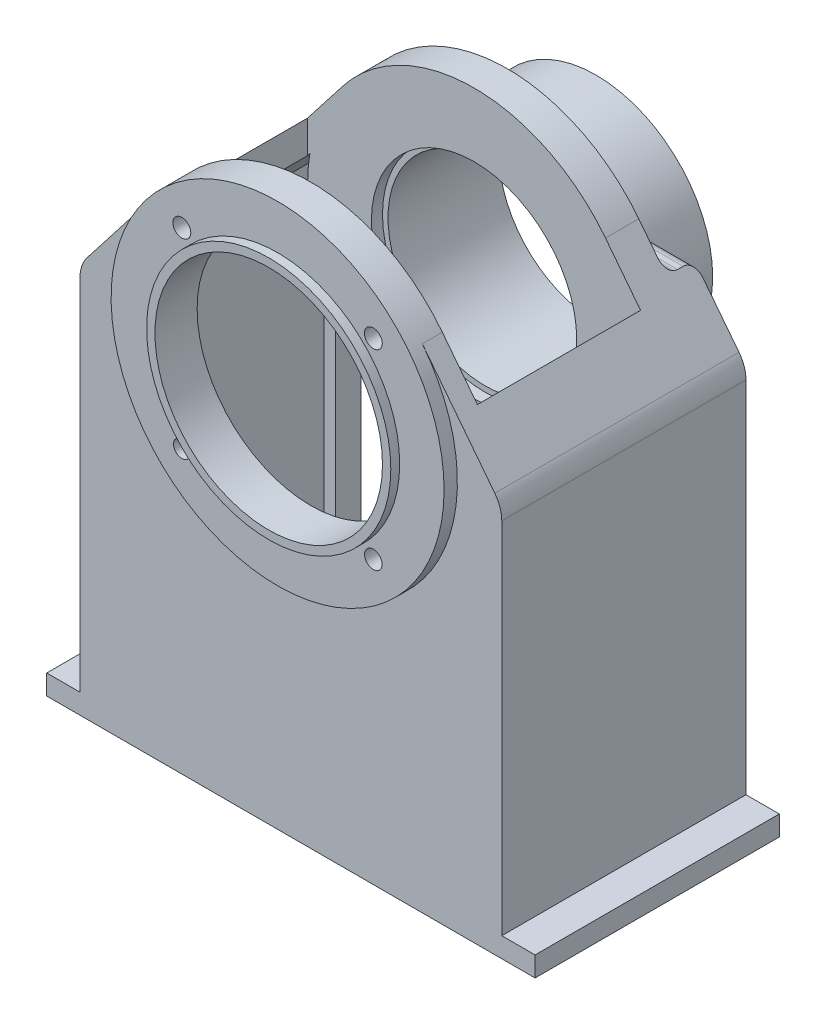
from build123d import *

# Parameters (mm, degrees)
BOSS_EXTRUDE1_DEPTH               = 7
SKETCH2_W                         = 48
SKETCH2_H                         = 7
BOSS_EXTRUDE2_DEPTH               = 352
SKETCH3_W                         = 18
SKETCH3_H                         = 7
BOSS_EXTRUDE3_DEPTH               = 352
BOSS_EXTRUDE4_DEPTH               = 18
BOSS_EXTRUDE5_START               = 30
BOSS_EXTRUDE5_DEPTH               = 30
BOSS_EXTRUDE6_DEPTH               = 147
BOSS_EXTRUDE7_DEPTH               = 147
BOSS_EXTRUDE8_START               = 18
BOSS_EXTRUDE8_DEPTH               = 18
SKETCH9_W                         = 30
SKETCH9_H                         = 220
CUT_EXTRUDE1_DEPTH                = 334
CUT_EXTRUDE2_DEPTH                = 30
CUT_EXTRUDE3_DEPTH                = 30
SKETCH12_W                        = 220
SKETCH12_H                        = 18
BOSS_EXTRUDE9_DEPTH               = 30
BOSS_EXTRUDE10_START              = 12
SKETCH13_R                        = 150
BOSS_EXTRUDE10_DEPTH              = 12
CUT_EXTRUDE4_DEPTH                = 37
SKETCH15_W                        = 340
SKETCH15_H                        = 240.614252285
BOSS_EXTRUDE11_DEPTH              = 5
CUT_EXTRUDE5_REACH                = 915.869
SKETCH16_W                        = 324
SKETCH16_H                        = 232.614252285
CUT_EXTRUDE6_DEPTH                = 25
SKETCH18_R                        = 110
BOSS_EXTRUDE12_DEPTH              = 8
SKETCH19_W                        = 105
SKETCH19_H                        = 80
HOLE1_D                           = 205
HOLE1_DEPTH                       = 38
M10_COUNTERBORE_HOLE1_D           = 12
M10_COUNTERBORE_HOLE1_DEPTH       = 45
M10_COUNTERBORE_HOLE1_CBORE_D     = 18
M10_COUNTERBORE_HOLE1_CBORE_DEPTH = 12
HOLE2_D                           = 175
HOLE2_CBORE_D                     = 185
HOLE2_CBORE_DEPTH                 = 10
FILLET1_R                         = 10
FILLET2_R                         = 18
FILLET3_R                         = 30
FILLET4_R                         = 150
SKETCH26_R                        = 8.054998693
SKETCH26_R_2                      = 7.927703382
SKETCH26_R_3                      = 7.509574851
CUT_EXTRUDE8_DEPTH                = 41


with BuildPart() as part:
    # Sketch1 → Boss-Extrude1 (new body)
    with BuildSketch(Plane.XY.offset(-1277.692981355)):
        with BuildLine():
            Line((671.230642584, 234.743963655), (711.230642584, 234.743963655))
            Line((711.230642584, 234.743963655), (521.230642584, 479.129447483))
            Line((521.230642584, 479.129447483), (331.230642584, 234.743963655))
            Line((331.230642584, 234.743963655), (371.230642584, 234.743963655))
            ThreePointArc((371.230642584, 234.743963655), (521.230642584, 84.743963655), (671.230642584, 234.743963655))
        make_face()
    extrude(amount=-BOSS_EXTRUDE1_DEPTH)

    # Sketch2 → Boss-Extrude2 (add)
    with BuildSketch(Plane.XZ.offset(-234.743963655)):
        with Locations((717.230642584, -1281.192981355)):
            Rectangle(SKETCH2_W, SKETCH2_H)
    extrude(amount=BOSS_EXTRUDE2_DEPTH)

    # Sketch3 → Boss-Extrude3 (add)
    with BuildSketch(Plane.XZ.offset(-234.743963654)):
        with Locations((340.230642584, -1281.192981355)):
            Rectangle(SKETCH3_W, SKETCH3_H)
    extrude(amount=BOSS_EXTRUDE3_DEPTH)

    # Sketch4 → Boss-Extrude4 (add)
    with BuildSketch(Plane(origin=(0, 0, -1284.692981355), x_dir=(-1, 0, 0), z_dir=(0, 0, -1))):
        Polygon((-331.230642584, -117.256036345), (-741.230642584, -117.256036345), (-741.230642584, 234.743963655), (-711.230642584, 234.743963655), (-521.230642584, 479.129447483), (-331.230642584, 234.743963655), align=None)
    extrude(amount=BOSS_EXTRUDE4_DEPTH)

    # Sketch5 → Boss-Extrude5 (add)
    with BuildSketch(Plane.XY.offset(-1277.692981355).offset(BOSS_EXTRUDE5_START)):
        with BuildLine():
            Line((371.230642584, 234.743963655), (354.030642584, 234.743963655))
            Line((354.030642584, 234.743963655), (349.230642584, 228.570014589))
            Line((349.230642584, 228.570014589), (349.230642584, -117.256036345))
            Line((349.230642584, -117.256036345), (331.230642584, -117.256036345))
            Line((331.230642584, -117.256036345), (331.230642584, 234.743963655))
            Line((331.230642584, 234.743963655), (521.230642584, 479.129447483))
            Line((521.230642584, 479.129447483), (711.230642584, 234.743963655))
            Line((711.230642584, 234.743963655), (741.230642584, 234.743963655))
            Line((741.230642584, 234.743963655), (741.230642584, -117.256036345))
            Line((741.230642584, -117.256036345), (693.230642584, -117.256036345))
            Line((693.230642584, -117.256036345), (693.230642584, 228.570014589))
            Line((693.230642584, 228.570014589), (688.430642584, 234.743963655))
            Line((688.430642584, 234.743963655), (671.230642584, 234.743963655))
            ThreePointArc((671.230642584, 234.743963655), (521.230642584, 84.743963655), (371.230642584, 234.743963655))
        make_face()
    extrude(amount=-BOSS_EXTRUDE5_DEPTH)

    # Sketch6 → Boss-Extrude6 (add)
    with BuildSketch(Plane.XY.offset(-1247.692981355)):
        Polygon((371.230642584, 256.867281138), (349.230642584, 228.570014589), (349.230642584, -117.256036345), (331.230642584, -117.256036345), (331.230642584, 234.743963655), (371.230642584, 286.193539197), align=None)
    extrude(amount=BOSS_EXTRUDE6_DEPTH)

    # Sketch7 → Boss-Extrude7 (add)
    with BuildSketch(Plane.XY.offset(-1247.692981355)):
        Polygon((741.230642584, -117.256036345), (693.230642584, -117.256036345), (693.230642584, 228.570014589), (671.230642584, 256.867281138), (671.230642584, 286.193539197), (711.230642584, 234.743963655), (741.230642584, 234.743963655), align=None)
    extrude(amount=BOSS_EXTRUDE7_DEPTH)

    # Sketch8 → Boss-Extrude8 (add)
    with BuildSketch(Plane.XY.offset(-1100.692981355).offset(BOSS_EXTRUDE8_START)):
        with BuildLine():
            Line((331.230642584, -117.256036345), (331.230642584, 234.743963654))
            Line((331.230642584, 234.743963654), (402.809589953, 326.811625152))
            ThreePointArc((402.809589953, 326.811625152), (521.230642584, 384.743963654), (639.651695216, 326.811625152))
            Line((639.651695216, 326.811625152), (711.230642584, 234.743963654))
            Line((711.230642584, 234.743963654), (741.230642584, 234.743963654))
            Line((741.230642584, 234.743963654), (741.230642584, -117.256036345))
            Line((741.230642584, -117.256036345), (331.230642584, -117.256036345))
        make_face()
    extrude(amount=-BOSS_EXTRUDE8_DEPTH)

    # Sketch9 → Cut-Extrude1 (cut)
    with BuildSketch(Plane(origin=(0, 234.743963655, 0), x_dir=(-1, 0, 0), z_dir=(0, 1, 0))):
        with Locations((-726.230642584, -1192.692981355)):
            Rectangle(SKETCH9_W, SKETCH9_H)
    extrude(amount=-CUT_EXTRUDE1_DEPTH, mode=Mode.SUBTRACT)

    # Sketch10 → Cut-Extrude2 (cut)
    with BuildSketch(Plane.XY.offset(-1247.692981355)):
        with BuildLine():
            Line((671.230642584, 234.743963655), (688.430642584, 234.743963655))
            Line((688.430642584, 234.743963655), (669.170885211, 259.516622202))
            ThreePointArc((669.170885211, 259.516622202), (670.714816319, 247.173034536), (671.230642584, 234.743963655))
        make_face()
    extrude(amount=-CUT_EXTRUDE2_DEPTH, mode=Mode.SUBTRACT)

    # Sketch11 → Cut-Extrude3 (cut)
    with BuildSketch(Plane.XY.offset(-1247.692981355)):
        with BuildLine():
            Line((373.290399958, 259.516622202), (354.030642584, 234.743963655))
            Line((354.030642584, 234.743963655), (371.230642584, 234.743963655))
            ThreePointArc((371.230642584, 234.743963655), (371.74646885, 247.173034536), (373.290399958, 259.516622202))
        make_face()
    extrude(amount=-CUT_EXTRUDE3_DEPTH, mode=Mode.SUBTRACT)

    # Sketch12 → Boss-Extrude9 (add)
    with BuildSketch(Plane.ZY.offset(-331.230642584)):
        with Locations((-1192.692981355, -108.256036346)):
            Rectangle(SKETCH12_W, SKETCH12_H)
    extrude(amount=BOSS_EXTRUDE9_DEPTH)

    # Sketch13 → Boss-Extrude10 (add)
    with BuildSketch(Plane.XY.offset(-1082.692981355).offset(BOSS_EXTRUDE10_START)):
        with Locations(Location((521.230642584, 234.743963655, 0), (0, 0, 142.136353638))):
            Circle(SKETCH13_R)
    extrude(amount=-BOSS_EXTRUDE10_DEPTH)

    # Sketch14 → Cut-Extrude4 (cut)
    with BuildSketch(Plane.XY.offset(-1247.692981355)):
        with BuildLine():
            Line((412.819587994, 184.743963655), (379.809286347, 184.743963655))
            ThreePointArc((379.809286347, 184.743963655), (521.230642584, 84.743963655), (662.651998822, 184.743963655))
            Line((662.651998822, 184.743963655), (629.641697174, 184.743963655))
            ThreePointArc((629.641697174, 184.743963655), (521.230642584, 115.35821594), (412.819587994, 184.743963655))
        make_face()
    extrude(amount=-CUT_EXTRUDE4_DEPTH, mode=Mode.SUBTRACT)

    # Sketch15 → Boss-Extrude11 (add)
    with BuildSketch(Plane(origin=(0, 0, -1302.692981355), x_dir=(-1, 0, 0), z_dir=(0, 0, -1))):
        with Locations((-521.230642584, 3.051089797)):
            Rectangle(SKETCH15_W, SKETCH15_H)
    extrude(amount=BOSS_EXTRUDE11_DEPTH)

    # Sketch16 → Cut-Extrude5 (cut, up to next)
    with BuildSketch(Plane(origin=(0, 0, -1307.692981355), x_dir=(-1, 0, 0), z_dir=(0, 0, -1)), mode=Mode.PRIVATE) as cut_extrude5_sk1:
        with Locations((-521.230642584, -0.948910203)):
            Rectangle(SKETCH16_W, SKETCH16_H)
    cut_extrude5_tool1 = extrude(cut_extrude5_sk1.sketch, amount=-CUT_EXTRUDE5_REACH, mode=Mode.PRIVATE) & part.part
    add(cut_extrude5_tool1.solids().sort_by_distance((521.230643, -0.94891, -1307.692981))[0], mode=Mode.SUBTRACT)

    # Sketch17 → Cut-Extrude6 (cut)
    with BuildSketch(Plane(origin=(0, 0, -1302.692981355), x_dir=(-1, 0, 0), z_dir=(0, 0, -1))):
        Polygon((-521.230642584, 479.129447483), (-664.583027426, 294.743963655), (-377.878257743, 294.743963655), align=None)
    extrude(amount=-CUT_EXTRUDE6_DEPTH, mode=Mode.SUBTRACT)

    # Sketch18 → Boss-Extrude12 (add)
    with BuildSketch(Plane.XY.offset(-1070.692981355)):
        with Locations((521.230642584, 234.743963655)):
            Circle(SKETCH18_R)
    extrude(amount=BOSS_EXTRUDE12_DEPTH)

    # Sketch19 → Revolve1 (revolve)
    with BuildSketch(Plane(origin=(280.2795082, 402.520798349, 0), x_dir=(-0.8206518066482866, 0.5714285714285761, 0), z_dir=(0.5714285714285761, 0.8206518066482866, 0)), mode=Mode.PRIVATE) as revolve1_sk:
        with Locations((-241.109460715, -1317.692981355)):
            Rectangle(SKETCH19_W, SKETCH19_H)
    revolve(revolve1_sk.sketch.rotate(Axis((521.230642584, 234.743963655, -1277.692981355), (0, 0, -1)), 325.150095421), axis=Axis((521.230642584, 234.743963655, -1277.692981355), (0, 0, -1)))

    # Hole1
    with Locations(Plane.XY.offset(-1062.692981355)):
        with Locations((521.230642584, 234.743963655)):
            Hole(HOLE1_D / 2, depth=HOLE1_DEPTH)

    # M10 counterbore hole1
    with Locations(Plane(origin=(0, 0, -1357.692981355), x_dir=(-1, 0, 0), z_dir=(0, 0, -1))):
        with Locations((-614.830642584, 234.743963655), (-521.230642584, 141.143963655), (-427.630642584, 234.743963655), (-521.230642584, 328.343963655)):
            CounterBoreHole(M10_COUNTERBORE_HOLE1_D / 2, M10_COUNTERBORE_HOLE1_CBORE_D / 2, M10_COUNTERBORE_HOLE1_CBORE_DEPTH, depth=M10_COUNTERBORE_HOLE1_DEPTH)

    # Hole2 (through all)
    with Locations(Plane.XY.offset(-1247.692981355)):
        with Locations((521.230642584, 234.743963655)):
            CounterBoreHole(HOLE2_D / 2, HOLE2_CBORE_D / 2, HOLE2_CBORE_DEPTH)

    # Fillet1
    fillet1_edges = [part.edges().sort_by_distance(p)[0] for p in [
        (683.230642584, 115.35821594, -1296.192981355),
        (359.230642584, 115.35821594, -1296.192981355),
        (635.991054854, 294.743963655, -1277.692981355),
        (635.991054854, 294.743963655, -1302.692981355),
        (406.470230315, 294.743963655, -1277.692981355),
        (406.470230315, 294.743963655, -1302.692981355),
    ]]
    fillet(fillet1_edges, radius=FILLET1_R)

    # Fillet2
    fillet2_edges = [part.edges().sort_by_distance(p)[0] for p in [
        (351.230642584, 123.35821594, -1305.192981355),
        (691.230642584, 123.35821594, -1305.192981355),
    ]]
    fillet(fillet2_edges, radius=FILLET2_R)

    # Fillet3
    fillet3_edges = [part.edges().sort_by_distance(p)[0] for p in [
        (331.230642584, 234.743963654, -1192.692981355),
        (711.230642584, 234.743963654, -1192.692981355),
    ]]
    fillet(fillet3_edges, radius=FILLET3_R)

    # Fillet4
    fillet4_edges = [part.edges().sort_by_distance(p)[0] for p in [
        (521.230642584, 479.129447483, -1262.692981355),
    ]]
    fillet(fillet4_edges, radius=FILLET4_R)

    # Sketch26 → Cut-Extrude8 (cut)
    with BuildSketch(Plane.XY.offset(-1070.692981355)):
        with Locations((434.96361528, 321.010990959)):
            Circle(SKETCH26_R)
        with Locations((607.497669889, 321.010990959)):
            Circle(SKETCH26_R)
        with Locations((607.497669889, 148.47693635)):
            Circle(SKETCH26_R_2)
        with Locations((434.96361528, 148.47693635)):
            Circle(SKETCH26_R_3)
    extrude(amount=-CUT_EXTRUDE8_DEPTH, mode=Mode.SUBTRACT)


solid = part.part
